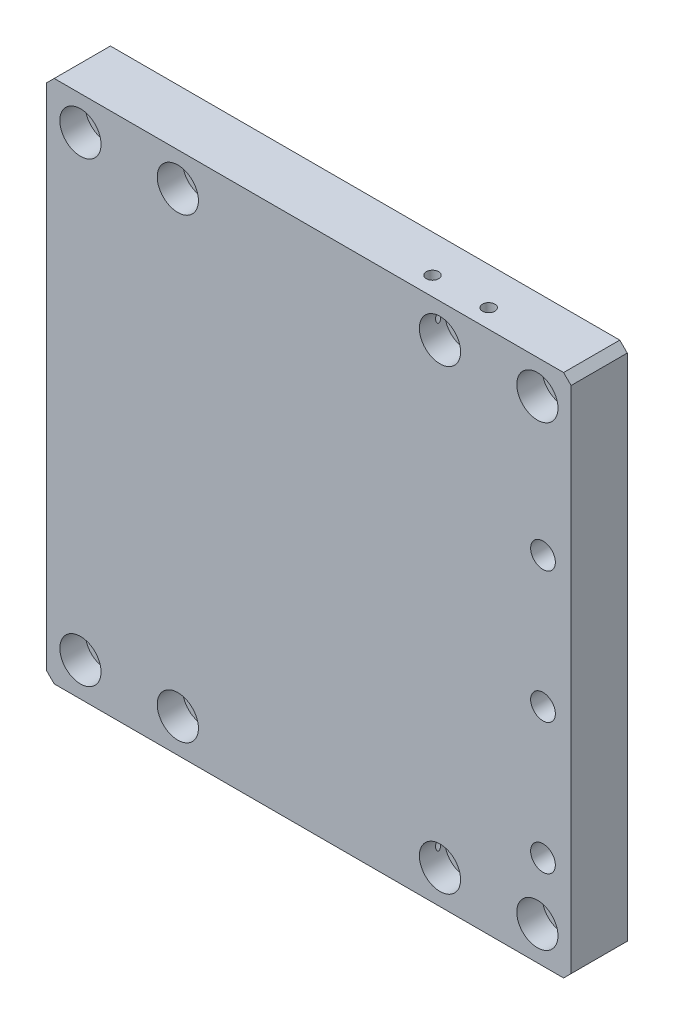
from build123d import *

# Parameters (mm, degrees)
SKETCH_1_W                  = 140
SKETCH_1_H                  = 140
EXTRUDE_1_DEPTH             = 15
HOLE_WIZARD_1_AT_2_COUNT    = 2
HOLE_WIZARD_1_AT_2_PITCH    = 26
HOLE_WIZARD_1_AT_3_COUNT    = 2
HOLE_WIZARD_1_AT_3_PITCH    = 96
HOLE_WIZARD_1_AT_4_COUNT    = 2
HOLE_WIZARD_1_AT_4_PITCH    = 122
PATTERN_LINEAR_1_COUNT      = 2
PATTERN_LINEAR_1_PITCH      = 122
HOLE_WIZARD_2_D             = 6.6
HOLE_WIZARD_2_CBORE_D       = 11
HOLE_WIZARD_2_CBORE_DEPTH   = 6.8
HOLE_WIZARD_M4_1_AT_2_COUNT = 2
HOLE_WIZARD_M4_1_AT_2_PITCH = 15
CHAMFER_1_SIZE              = 2


with BuildPart() as part:
    # 草图1 → 凸台-拉伸1 (new body)
    with BuildSketch(Plane.XY):
        Rectangle(SKETCH_1_W, SKETCH_1_H)
    extrude(amount=EXTRUDE_1_DEPTH)

    # 草图2 → 打孔尺寸(%根据)内六角圆柱头螺钉的类型1 (revolve, cut)
    with BuildSketch(Plane(origin=(-61, 61, 15), x_dir=(0, -1, 0), z_dir=(1, 0, 0))):
        Polygon((0, 0), (0, 16.982840043), (3.3, 15), (3.3, 6.8), (5.5, 6.8), (5.5, 0), align=None)
    hole_wizard_1 = revolve(axis=Axis((-61, 61, 21.35), (0, 0, -1)), mode=Mode.SUBTRACT)

    # 打孔尺寸(%根据)内六角圆柱头螺钉的类型1 at 2: 打孔尺寸(%根据)内六角圆柱头螺钉的类型1 ×2
    with Locations(*[(i * HOLE_WIZARD_1_AT_2_PITCH, 0, 0) for i in range(1, HOLE_WIZARD_1_AT_2_COUNT)]):
        add(hole_wizard_1, mode=Mode.SUBTRACT)

    # 打孔尺寸(%根据)内六角圆柱头螺钉的类型1 at 3: 打孔尺寸(%根据)内六角圆柱头螺钉的类型1 ×2
    with Locations(*[(i * HOLE_WIZARD_1_AT_3_PITCH, 0, 0) for i in range(1, HOLE_WIZARD_1_AT_3_COUNT)]):
        add(hole_wizard_1, mode=Mode.SUBTRACT)

    # 打孔尺寸(%根据)内六角圆柱头螺钉的类型1 at 4: 打孔尺寸(%根据)内六角圆柱头螺钉的类型1 ×2
    with Locations(*[(i * HOLE_WIZARD_1_AT_4_PITCH, 0, 0) for i in range(1, HOLE_WIZARD_1_AT_4_COUNT)]):
        add(hole_wizard_1, mode=Mode.SUBTRACT)

    # 阵列(线性)1: 打孔尺寸(%根据)内六角圆柱头螺钉的类型1 ×2
    with Locations(*[(0, -i * PATTERN_LINEAR_1_PITCH, 0) for i in range(1, PATTERN_LINEAR_1_COUNT)]):
        add(hole_wizard_1, mode=Mode.SUBTRACT)

    # 阵列(线性)1 copy 1 sketch → 阵列(线性)1 copy 1 (revolve, cut)
    with BuildSketch(Plane(origin=(-35, -61, 15), x_dir=(0, -1, 0), z_dir=(1, 0, 0))):
        Polygon((0, 0), (0, 16.982840043), (3.3, 15), (3.3, 6.8), (5.5, 6.8), (5.5, 0), align=None)
    revolve(axis=Axis((-35, -61, 21.35), (0, 0, -1)), mode=Mode.SUBTRACT)

    # 阵列(线性)1 copy 2 sketch → 阵列(线性)1 copy 2 (revolve, cut)
    with BuildSketch(Plane(origin=(35, -61, 15), x_dir=(0, -1, 0), z_dir=(1, 0, 0))):
        Polygon((0, 0), (0, 16.982840043), (3.3, 15), (3.3, 6.8), (5.5, 6.8), (5.5, 0), align=None)
    revolve(axis=Axis((35, -61, 21.35), (0, 0, -1)), mode=Mode.SUBTRACT)

    # 阵列(线性)1 copy 3 sketch → 阵列(线性)1 copy 3 (revolve, cut)
    with BuildSketch(Plane(origin=(61, -61, 15), x_dir=(0, -1, 0), z_dir=(1, 0, 0))):
        Polygon((0, 0), (0, 16.982840043), (3.3, 15), (3.3, 6.8), (5.5, 6.8), (5.5, 0), align=None)
    revolve(axis=Axis((61, -61, 21.35), (0, 0, -1)), mode=Mode.SUBTRACT)

    # 打孔尺寸(%根据)内六角圆柱头螺钉的类型2 (through all)
    with Locations(Plane(origin=(0, 0, 0), x_dir=(-1, 0, 0), z_dir=(0, 0, -1))):
        with Locations((-62.5, 25), (-62.5, -10), (-62.5, -45)):
            CounterBoreHole(HOLE_WIZARD_2_D / 2, HOLE_WIZARD_2_CBORE_D / 2, HOLE_WIZARD_2_CBORE_DEPTH)

    # 草图7 → M4 螺纹孔1 (revolve, cut)
    with BuildSketch(Plane(origin=(28, 70, 10), x_dir=(0, 0, 1), z_dir=(1, 0, 0))):
        Polygon((0, 0), (0, 15.091420021), (1.65, 14.1), (1.65, 0), align=None)
    hole_wizard_m4_1 = revolve(axis=Axis((28, 76.35, 10), (0, -1, 0)), mode=Mode.SUBTRACT)

    # M4 螺纹孔1 at 2: M4 螺纹孔1 ×2
    with Locations(*[(i * HOLE_WIZARD_M4_1_AT_2_PITCH, 0, 0) for i in range(1, HOLE_WIZARD_M4_1_AT_2_COUNT)]):
        add(hole_wizard_m4_1, mode=Mode.SUBTRACT)

    # 倒角1
    chamfer_1_edges = [part.edges().sort_by_distance(p)[0] for p in [
        (70, -70, 7.5),
        (-70, -70, 7.5),
        (-70, 70, 7.5),
        (70, 70, 7.5),
    ]]
    chamfer(chamfer_1_edges, length=CHAMFER_1_SIZE)

    # 镜向1: M4 螺纹孔1 across plane
    add(hole_wizard_m4_1.mirror(Plane.ZX), mode=Mode.SUBTRACT)

    # 镜向1 copy 1 sketch → 镜向1 copy 1 (revolve, cut)
    with BuildSketch(Plane(origin=(43, -70, 10), x_dir=(0, 0, 1), z_dir=(1, 0, 0))):
        Polygon((0, 0), (0, -15.091420021), (1.65, -14.1), (1.65, 0), align=None)
    revolve(axis=Axis((43, -76.35, 10), (0, -1, 0)), mode=Mode.SUBTRACT)


solid = part.part
